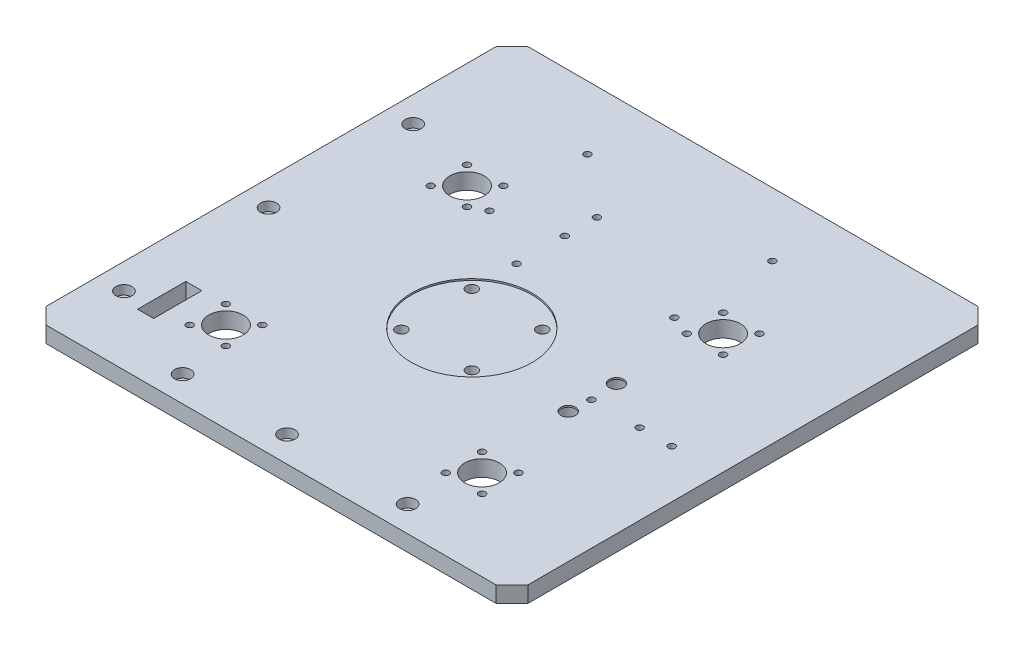
from build123d import *

# Parameters (mm, degrees)
SKETCH1_W                                            = 300
SKETCH1_H                                            = 300
BOSS_EXTRUDE1_DEPTH                                  = 10
SKETCH2_R                                            = 37.5
CUT_EXTRUDE1_DEPTH                                   = 1
SKETCH3_W                                            = 10
SKETCH3_H                                            = 30
CUT_EXTRUDE2_DEPTH                                   = 213.367605816
SKETCH4_R                                            = 10.75
CUT_EXTRUDE3_DEPTH                                   = 213.367605816
CBORE_FOR_M8_HEXAGON_SOCKET_HEAD_CAP_SCR_D           = 9
CBORE_FOR_M8_HEXAGON_SOCKET_HEAD_CAP_SCR_CBORE_D     = 15
CBORE_FOR_M8_HEXAGON_SOCKET_HEAD_CAP_SCR_CBORE_DEPTH = 9
M8_TAPPED_HOLE1_D                                    = 6.8
M5_TAPPED_HOLE1_D                                    = 4.2
M5_TAPPED_HOLE2_D                                    = 4.2
CHAMFER1_SIZE                                        = 10
M5_TAPPED_HOLE3_D                                    = 4.2
M5_TAPPED_HOLE3_DEPTH                                = 36.9
M5_TAPPED_HOLE3_TIP                                  = 1.2618073
CBORE_FOR_M5_HEXAGON_SOCKET_HEAD_CAP_SCR_D           = 5.5
CBORE_FOR_M5_HEXAGON_SOCKET_HEAD_CAP_SCR_DEPTH       = 36.9
CBORE_FOR_M5_HEXAGON_SOCKET_HEAD_CAP_SCR_CBORE_D     = 10
CBORE_FOR_M5_HEXAGON_SOCKET_HEAD_CAP_SCR_CBORE_DEPTH = 5.7
CBORE_FOR_M5_HEXAGON_SOCKET_HEAD_CAP_SCR_TIP         = 1.652366702


with BuildPart() as part:
    # Sketch1 → Boss-Extrude1 (new body)
    with BuildSketch(Plane(origin=(0, 0, 0), x_dir=(1, 0, 0), z_dir=(0, 1, 0))):
        Rectangle(SKETCH1_W, SKETCH1_H)
    extrude(amount=BOSS_EXTRUDE1_DEPTH)

    # Sketch2 → Cut-Extrude1 (cut)
    with BuildSketch(Plane(origin=(0, 10, 0), x_dir=(1, 0, 0), z_dir=(0, 1, 0))):
        with Locations(Location((-6, -19, 0), (0, 0, 270))):
            Circle(SKETCH2_R)
    extrude(amount=-CUT_EXTRUDE1_DEPTH, mode=Mode.SUBTRACT)

    # Sketch3 → Cut-Extrude2 (cut, through all)
    with BuildSketch(Plane(origin=(0, 10, 0), x_dir=(1, 0, 0), z_dir=(0, 1, 0))):
        with Locations((-115, -98)):
            Rectangle(SKETCH3_W, SKETCH3_H)
    extrude(amount=-CUT_EXTRUDE2_DEPTH, mode=Mode.SUBTRACT)

    # Sketch4 → Cut-Extrude3 (cut, through all)
    with BuildSketch(Plane(origin=(0, 10, 0), x_dir=(1, 0, 0), z_dir=(0, 1, 0))):
        with Locations(Location((-84, -94, 0), (0, 0, 270))):
            Circle(SKETCH4_R)
        with Locations(Location((-84, 56, 0), (0, 0, 270))):
            Circle(SKETCH4_R)
        with Locations(Location((75.36030205, 56, 0), (0, 0, 270))):
            Circle(SKETCH4_R)
        with Locations(Location((75.36030205, -94, 0), (0, 0, 270))):
            Circle(SKETCH4_R)
    extrude(amount=-CUT_EXTRUDE3_DEPTH, mode=Mode.SUBTRACT)

    # CBORE for M8 Hexagon socket head cap screws1 (through all)
    with Locations(Plane(origin=(0, 0, 0), x_dir=(-1, 0, 0), z_dir=(0, -1, 0))):
        with Locations((-69, -4), (-69, -34)):
            CounterBoreHole(CBORE_FOR_M8_HEXAGON_SOCKET_HEAD_CAP_SCR_D / 2, CBORE_FOR_M8_HEXAGON_SOCKET_HEAD_CAP_SCR_CBORE_D / 2, CBORE_FOR_M8_HEXAGON_SOCKET_HEAD_CAP_SCR_CBORE_DEPTH)

    # M8 Tapped Hole1 (through all)
    with Locations(Plane(origin=(0, 10, 0), x_dir=(1, 0, 0), z_dir=(0, 1, 0))):
        with Locations((15.922198881, -40.918421389), (15.918421389, 2.922198881), (-27.922198881, 2.918421389), (-27.918421389, -40.922198881)):
            Hole(M8_TAPPED_HOLE1_D / 2)

    # M5 Tapped Hole1 (through all)
    with Locations(Plane(origin=(0, 0, 0), x_dir=(-1, 0, 0), z_dir=(0, -1, 0))):
        with Locations((72.686291501, 44.686291501), (95.313708499, 44.686291501), (95.313708499, 67.313708499), (72.686291501, 67.313708499), (95.313708499, -82.686291501), (95.313708499, -105.313708499), (72.686291501, -105.313708499), (72.686291501, -82.686291501), (-64.046593551, -82.686291501), (-64.046593551, -105.313708499), (-86.674010549, -105.313708499), (-86.674010549, -82.686291501), (-64.046593551, 67.313708499), (-64.046593551, 44.686291501), (-86.674010549, 44.686291501), (-86.674010549, 67.313708499)):
            Hole(M5_TAPPED_HOLE1_D / 2)

    # M5 Tapped Hole2 (through all)
    with Locations(Plane(origin=(0, 10, 0), x_dir=(1, 0, 0), z_dir=(0, 1, 0))):
        with Locations((51.55, 110.5), (-63.55, 110.5), (-63.55, 49.5), (51.55, 49.5)):
            Hole(M5_TAPPED_HOLE2_D / 2)

    # Chamfer1
    chamfer1_edges = [part.edges().sort_by_distance(p)[0] for p in [
        (150, 5, 150),
        (-150, 5, 150),
        (-150, 5, -150),
        (150, 5, -150),
    ]]
    chamfer(chamfer1_edges, length=CHAMFER1_SIZE)

    # M5 Tapped Hole3
    with Locations(Plane(origin=(0, 0, 0), x_dir=(-1, 0, 0), z_dir=(0, -1, 0))):
        with Locations((26.578080425, 59.413568319), (-100, -20.593013208), (26.578080425, 79.413568319), (26.578080425, 29.413568319), (-120, -20.593013208), (-70, -20.593013208)):
            Hole(M5_TAPPED_HOLE3_D / 2, depth=M5_TAPPED_HOLE3_DEPTH)
            with Locations((0, 0, -(M5_TAPPED_HOLE3_DEPTH + M5_TAPPED_HOLE3_TIP / 2))):  # 118° drill point
                Cone(0, M5_TAPPED_HOLE3_D / 2, M5_TAPPED_HOLE3_TIP, mode=Mode.SUBTRACT)

    # CBORE for M5 Hexagon socket head cap screws1
    with Locations(Plane(origin=(0, 10, 0), x_dir=(1, 0, 0), z_dir=(0, 1, 0))):
        with Locations((-134, -107.5), (-71, -134), (-6, -134), (69, -134), (-134, 72.5), (-134, -17.5)):
            CounterBoreHole(CBORE_FOR_M5_HEXAGON_SOCKET_HEAD_CAP_SCR_D / 2, CBORE_FOR_M5_HEXAGON_SOCKET_HEAD_CAP_SCR_CBORE_D / 2, CBORE_FOR_M5_HEXAGON_SOCKET_HEAD_CAP_SCR_CBORE_DEPTH, depth=CBORE_FOR_M5_HEXAGON_SOCKET_HEAD_CAP_SCR_DEPTH)
            with Locations((0, 0, -(CBORE_FOR_M5_HEXAGON_SOCKET_HEAD_CAP_SCR_DEPTH + CBORE_FOR_M5_HEXAGON_SOCKET_HEAD_CAP_SCR_TIP / 2))):  # 118° drill point
                Cone(0, CBORE_FOR_M5_HEXAGON_SOCKET_HEAD_CAP_SCR_D / 2, CBORE_FOR_M5_HEXAGON_SOCKET_HEAD_CAP_SCR_TIP, mode=Mode.SUBTRACT)


solid = part.part
